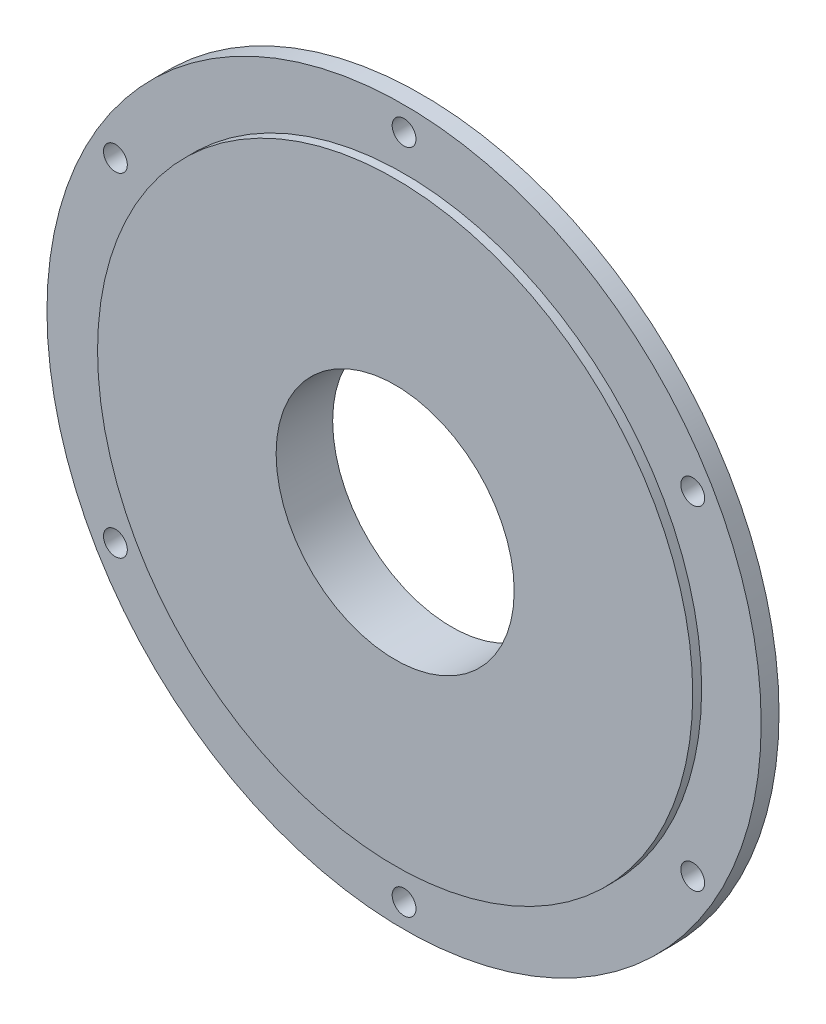
from build123d import *

# Parameters (mm, degrees)
SKETCH2_R          = 2
CUT_EXTRUDE1_DEPTH = 10


with BuildPart() as part:
    # Sketch1 → Revolve1 (revolve)
    with BuildSketch(Plane(origin=(0, 0, 0), x_dir=(1, 0, 0), z_dir=(0, 1, 0)), mode=Mode.PRIVATE) as revolve1_sk:
        Polygon((20, 9.5), (20, 0), (50, 0), (50, 1.5), (60, 1.5), (60, 4.5), (23, 4.5), (23, 9.5), align=None)
    revolve(revolve1_sk.sketch.rotate(Axis((0, 0, -4.956904689), (0, 0, 1)), 180), axis=Axis((0, 0, -4.956904689), (0, 0, 1)))

    # Sketch2 → Cut-Extrude1 (cut)
    with BuildSketch(Plane(origin=(0, 0, -4.5), x_dir=(-1, 0, 0), z_dir=(0, 0, -1))):
        with Locations((0, 56)):
            Circle(SKETCH2_R)
        with Locations((-48.497422612, 28)):
            Circle(SKETCH2_R)
        with Locations((-48.497422612, -28)):
            Circle(SKETCH2_R)
        with Locations((0, -56)):
            Circle(SKETCH2_R)
        with Locations((48.497422612, -28)):
            Circle(SKETCH2_R)
        with Locations((48.497422612, 28)):
            Circle(SKETCH2_R)
    extrude(amount=-CUT_EXTRUDE1_DEPTH, mode=Mode.SUBTRACT)


solid = part.part
